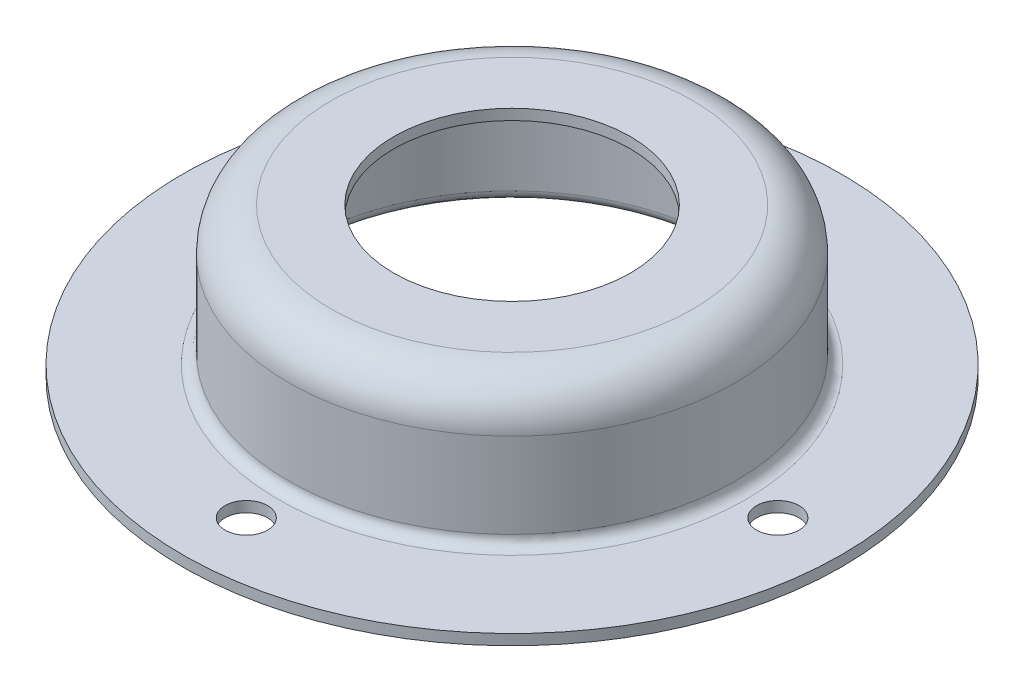
from build123d import *

# Parameters (mm, degrees)
SKETCH_2_R          = 2
CUT_EXTRUDE_1_DEPTH = 1
SKETCH_3_R          = 11.13
CUT_EXTRUDE_2_DEPTH = 10


with BuildPart() as part:
    # 草图1 → 旋转3 (revolve)
    with BuildSketch(Plane.XY):
        with BuildLine():
            Line((0, 13), (0, 12))
            Line((0, 12), (16, 12))
            ThreePointArc((16, 12), (18.828427125, 10.828427125), (20, 8))
            Line((20, 8), (20, 0))
            ThreePointArc((20, 0), (20.292893219, -0.707106781), (21, -1))
            Line((21, -1), (31, -1))
            Line((31, -1), (31, 0))
            Line((31, 0), (22, 0))
            ThreePointArc((22, 0), (21.292893219, 0.292893219), (21, 1))
            Line((21, 1), (21, 9))
            ThreePointArc((21, 9), (19.828427125, 11.828427125), (17, 13))
            Line((17, 13), (0, 13))
        make_face()
    revolve(axis=Axis((0, 0, 0), (0, 1, 0)))

    # 草图2 → 切除-拉伸1 (cut)
    with BuildSketch(Plane(origin=(0, 0, 0), x_dir=(1, 0, 0), z_dir=(0, 1, 0))):
        with Locations(Location((0, 25, 0), (0, 0, 180))):
            Circle(SKETCH_2_R)
        with Locations(Location((25, 0, 0), (0, 0, 180))):
            Circle(SKETCH_2_R)
        with Locations(Location((0, -25, 0), (0, 0, 180))):
            Circle(SKETCH_2_R)
        with Locations(Location((-25, 0, 0), (0, 0, 180))):
            Circle(SKETCH_2_R)
    extrude(amount=-CUT_EXTRUDE_1_DEPTH, mode=Mode.SUBTRACT)

    # 草图3 → 切除-拉伸2 (cut)
    with BuildSketch(Plane(origin=(0, 13, 0), x_dir=(1, 0, 0), z_dir=(0, 1, 0))):
        with Locations(Location((0, 0, 0), (0, 0, 180))):
            Circle(SKETCH_3_R)
    extrude(amount=-CUT_EXTRUDE_2_DEPTH, mode=Mode.SUBTRACT)


solid = part.part
